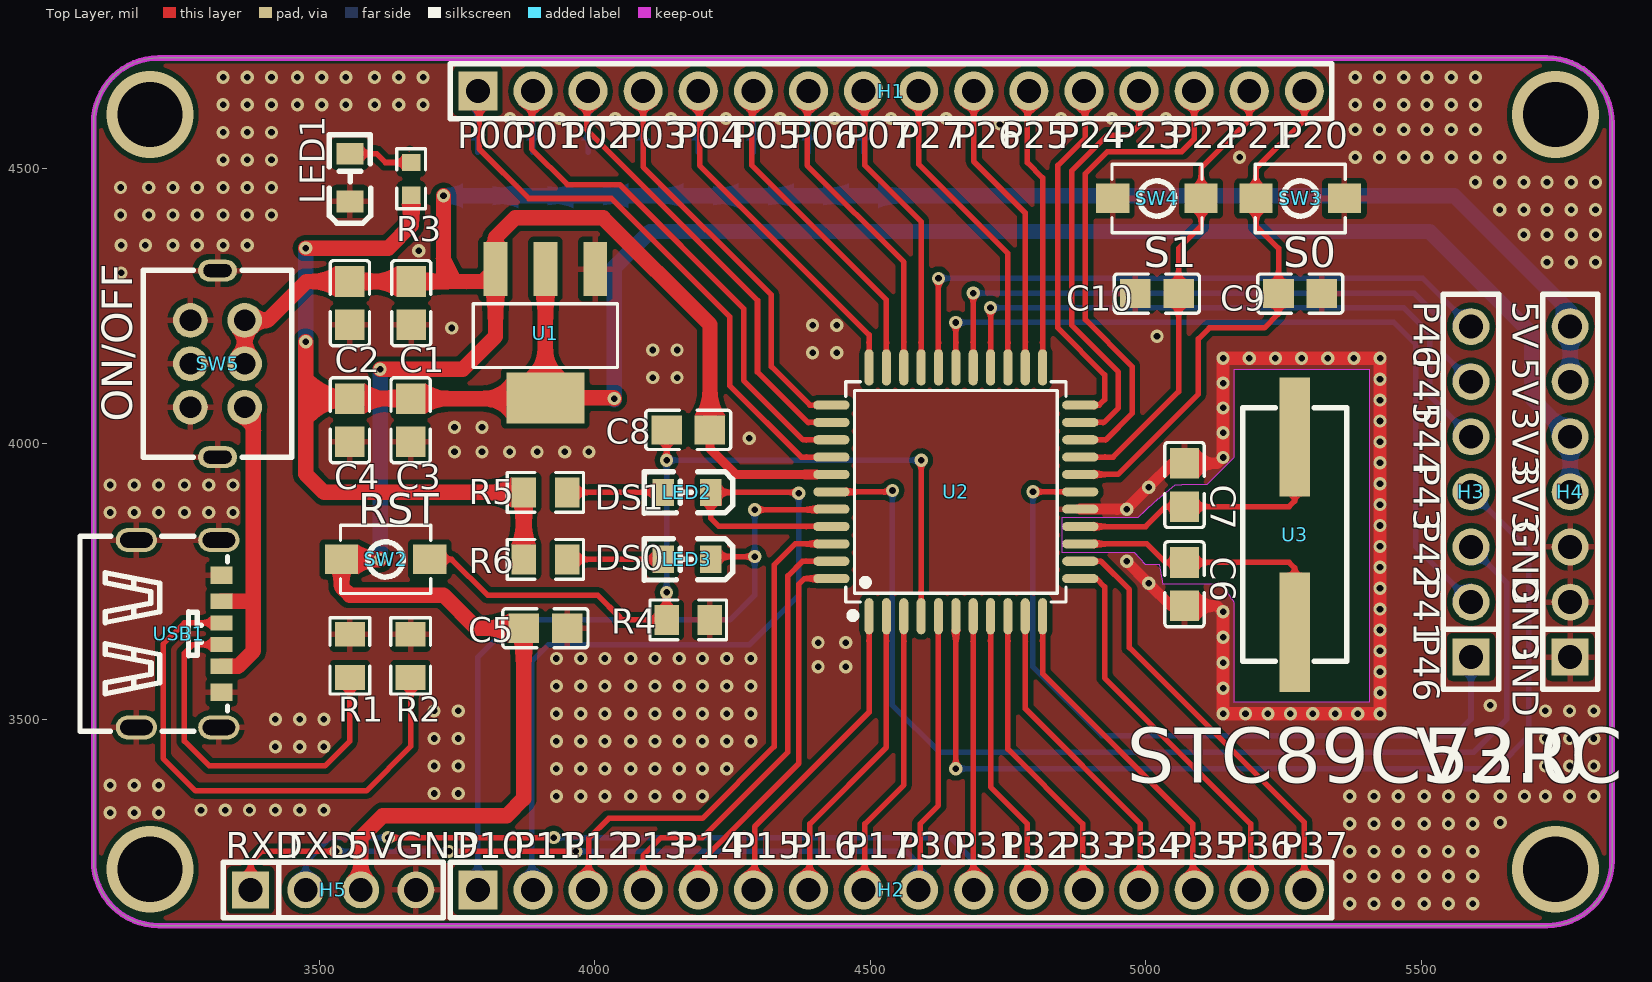
[diagram p0: Top Layer view]
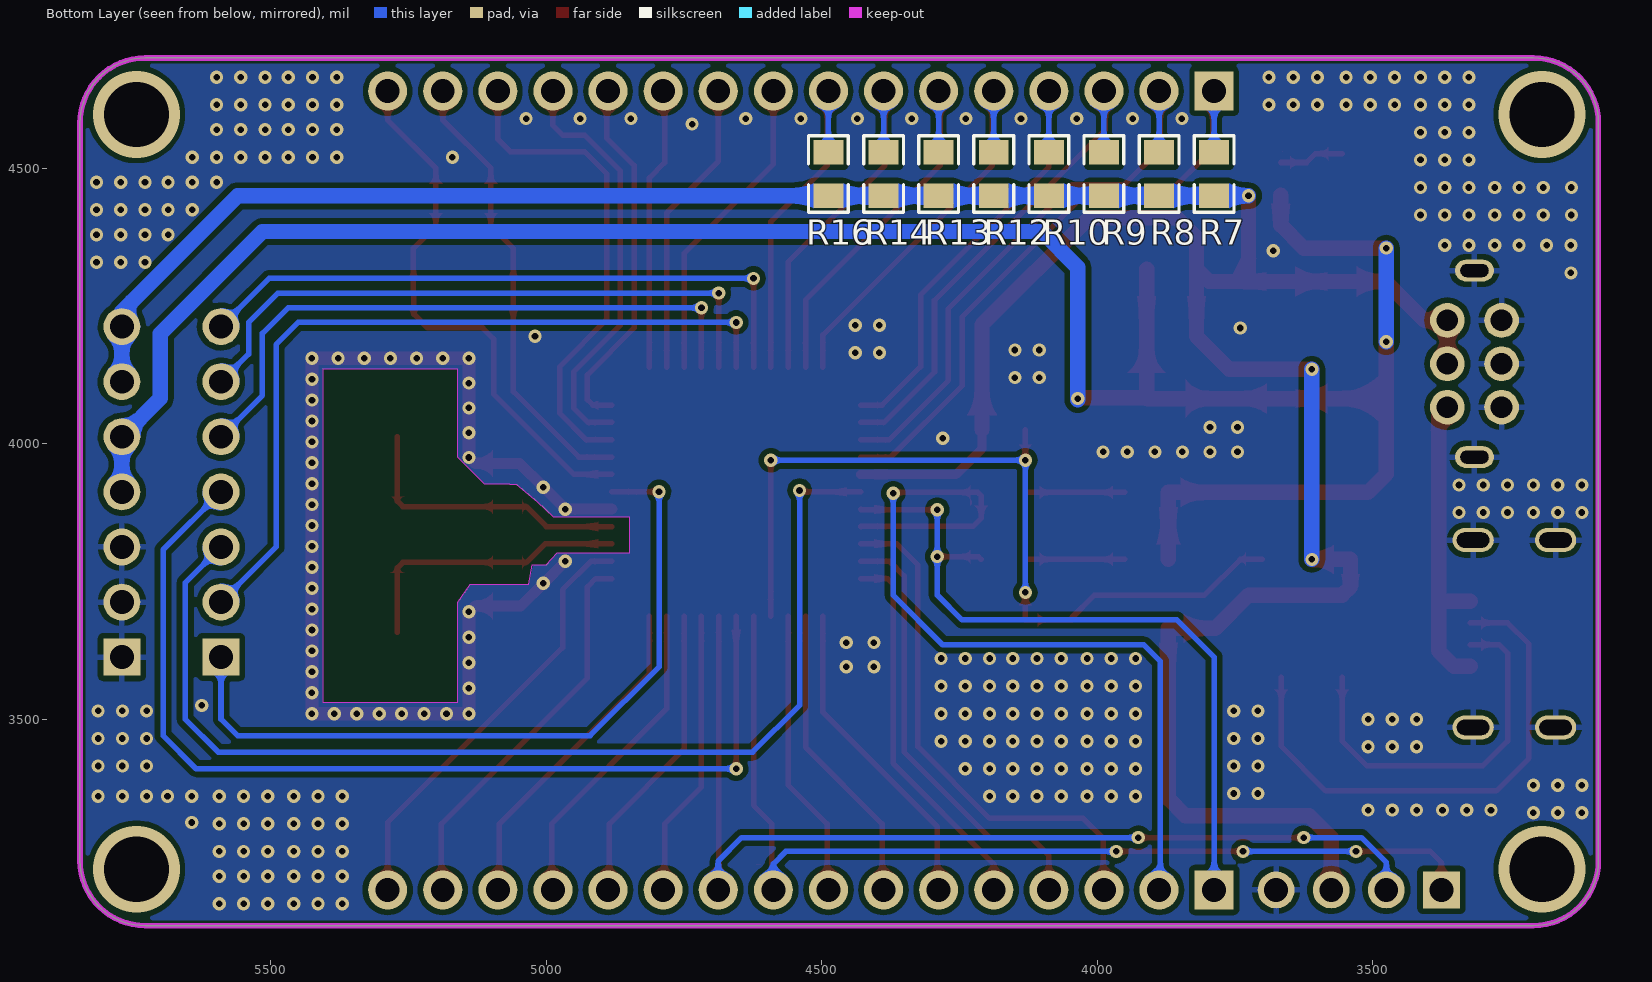
[diagram p1: Bottom Layer view, seen from below]
# Altium PCB MISC51716.pcbdoc
Units mil, origin at the board's own origin, x right, y up, seen from the top; angles counter-clockwise.
Board outline 2755.91 x 1574.8 mil, 2 copper layers (Top Layer, Bottom Layer), stack 62.206 mil thick; 40 components, 52 nets, 178 pads, 332 vias.

## Layer stack, top to bottom
Top Solder Mask Layer: solder mask 0.394, Dk 3.3
Top Layer: signal copper 1.379
Dielectric1: surface 59.449, FR4, Dk 4.5
Bottom Layer: signal copper 1.378
Bottom Solder Mask Layer: solder mask 0.394, Dk 3.3

## Board outline
3208.11,4700 ccw(c3208.11,4581.89) 3090,4581.89 3090,3243.31 ccw(c3208.11,3243.31) 3208.11,3125.2 5727.8,3125.2 ccw(c5727.8,3243.31) 5845.91,3243.31 5845.91,4581.89 ccw(c5727.8,4581.89) 5727.8,4700

## Design rules (kind name [scope] priority, off if disabled: settings)
BoardOutlineClearance copperThickness2oz_1 [All] p2 off: genericclearance=7.99 ignorepadtopadclearanceinfootprint=FALSE except(0: Arc-SplitContinuation Track-SplitContinuation SMDPad-SplitContinuation THPad-SplitContinuation Via-SplitContinuation Fill-SplitContinuation Region-SplitContinuation Poly-SplitContinuation Text-SplitContinuation Hole-SplitContinuation; 5.98: Arc-CutoutEdge SMDPad-CutoutEdge THPad-CutoutEdge Via-CutoutEdge Fill-CutoutEdge Region-CutoutEdge Text-CutoutEdge; 6.93: Hole-OutlineEdge Hole-CutoutEdge; 10: Poly-OutlineEdge Poly-CutoutEdge; 11.81: Arc-OutlineEdge Track-OutlineEdge SMDPad-OutlineEdge THPad-OutlineEdge Via-OutlineEdge Fill-OutlineEdge Region-OutlineEdge Text-OutlineEdge Track-CutoutEdge)
BoardOutlineClearance copperThickness1oz_1 [All] p4: genericclearance=4.02 ignorepadtopadclearanceinfootprint=FALSE except(0: Arc-SplitContinuation Track-SplitContinuation SMDPad-SplitContinuation THPad-SplitContinuation Via-SplitContinuation Fill-SplitContinuation Region-SplitContinuation Poly-SplitContinuation Text-SplitContinuation Hole-SplitContinuation; 6: SMDPad-CutoutEdge THPad-CutoutEdge Via-CutoutEdge Fill-CutoutEdge Region-CutoutEdge Text-CutoutEdge; 6.93: Hole-OutlineEdge Hole-CutoutEdge; 10: Poly-OutlineEdge Poly-CutoutEdge; 11.8: Arc-OutlineEdge Track-OutlineEdge SMDPad-OutlineEdge THPad-OutlineEdge Via-OutlineEdge Fill-OutlineEdge Region-OutlineEdge Text-OutlineEdge; 11.81: Arc-CutoutEdge Track-CutoutEdge)
Clearance copperThickness2oz [All] p1 off: gap=7.99 ignorepadtopadclearanceinfootprint=FALSE except(5.98: SMDPad-Track SMDPad-SMDPad THPad-Track SMDPad-THPad THPad-THPad Track-Via SMDPad-Via THPad-Via Via-Via Fill-Track Region-Track Fill-SMDPad Region-SMDPad Fill-THPad Region-THPad Fill-Via Region-Via Fill-Fill Fill-Region Region-Region Arc-Track Arc-SMDPad Arc-THPad Arc-Via Fill-Arc Region-Arc Arc-Arc Text-Track SMDPad-Text Text-THPad Text-Via Fill-Text Region-Text Arc-Text Text-Text; 6.93: Hole-Track Hole-SMDPad Hole-THPad Hole-Via Fill-Hole Region-Hole Hole-Arc Hole-Text; 10: Poly-Track Poly-SMDPad Poly-THPad Poly-Via Poly-Fill Poly-Region Poly-Poly Poly-Arc Poly-Text Poly-Hole)
Clearance copperThickness1oz [All] p3: gap=4.02 ignorepadtopadclearanceinfootprint=FALSE except(5.98: SMDPad-Track SMDPad-SMDPad THPad-Track SMDPad-THPad THPad-THPad Track-Via SMDPad-Via THPad-Via Via-Via Fill-Track Region-Track Fill-SMDPad Region-SMDPad Fill-THPad Region-THPad Fill-Via Region-Via Fill-Fill Fill-Region Region-Region; 6: Arc-Track Arc-SMDPad Arc-THPad Arc-Via Fill-Arc Region-Arc Arc-Arc Text-Track SMDPad-Text Text-THPad Text-Via Fill-Text Region-Text Arc-Text Text-Text; 6.93: Hole-Track Hole-SMDPad Hole-THPad Hole-Via Fill-Hole Region-Hole Hole-Arc Hole-Text; 10: Poly-Track Poly-SMDPad Poly-THPad Poly-Via Poly-Fill Poly-Region Poly-Poly Poly-Arc Poly-Text Poly-Hole)
Creepage creepage [All] p1: checkdistance=0 ignoreinternallayers=TRUE applytopolygonpour=TRUE
DiffPairsRouting differentialPair [All] p1: maxlimit=6 minlimit=6 mostfreqgap=6 toplayer_minwidth=5 toplayer_prefwidth=10 toplayer_maxwidth=100 toplayer_mingap=6 toplayer_prefgap=6 toplayer_maxgap=6 bottomlayer_minwidth=5 bottomlayer_prefwidth=10 bottomlayer_maxwidth=100 bottomlayer_mingap=6 bottomlayer_prefgap=6 bottomlayer_maxgap=6 maxuncoupledlength=10
HoleToHoleClearance otherClearance [All] p1: gap=11.81 allowstackedmicrovias=TRUE
Length netLength [All] p1: minlimit=0 maxlimit=0
MatchedLengths netLengthTolerance [All] p1: tolerance=1000
PasteMaskExpansion pasteMaskExpansion [All] p1: expansion=0
PlaneConnect innerPlane [All] p1: planeconnectstyle=Relief reliefexpansion=20 reliefentries=4 reliefconductorwidth=10 reliefairgap=10
PolygonConnect copperRegion [All] p1: connectstyle=Relief reliefconductorwidth=10 reliefentries=4 polygonreliefangle="90 Angle" airgapwidth=10 via.connectstyle=Relief via.reliefconductorwidth=10 via.reliefentries=4 via.polygonreliefangle="90 Angle" via.airgapwidth=10
RoutingVias viaSize [All] p1: holewidth=12.01 width=24.02 viastyle="Through Hole" minholewidth=11.81 minwidth=19.68 maxholewidth=248.03 maxwidth=393.7
SolderMaskExpansion solderMaskExpansion [IsVia] p1: expansion=-1000 istentingtop=TRUE
SolderMaskExpansion solderMaskExpansion [All] p2: expansion=2 istentingtop=FALSE
Width copperThickness2oz_2 [All] p1 off: maxlimit=100 minlimit=8 preferedwidth=10
Width copperThickness1oz_2 [All] p2: maxlimit=100 minlimit=5 preferedwidth=10

## Components (designator, comment, footprint, x,y, rotation, side; value= is the part's Value field where it differs from the comment)
C1 "100nF" C0805 3666.52,4255 r90 top
C2 "10UF" C0805 3555.15,4255 r90 top
C3 "100nF" C0805 3665.49,4042.5 r90 top
C4 "10UF" C0805 3555.15,4042.5 r90 top
C5 "100nF" C0805 3910,3665 r180 top
C6 "47PF" C0805 5070,3745 r270 top
C7 "47PF" C0805 5070,3925 r90 top
C8 "10UF" C0805 4169.33,4025 r180 top
C9 "10UF" C0805 5280,4272.5 r180 top
C10 "10UF" C0805 5020,4272.5 r0 top
H1 "" HDR-TH_16P-P2.54-V-M 4537.5,4640 r0 top
H2 "" HDR-TH_16P-P2.54-V-M 4537.5,3190 r0 top
H3 "" HDR-TH_7P-P2.54-V-M 5590,3912.5 r90 top
H4 "" HDR-TH_7P-P2.54-V-M 5770,3912.5 r90 top
H5 "" HDR-TH_4P-P2.54-V-M 3525,3190 r0 top
LED1 "" LED_0805 3555.55,4485 r90 top
LED2 "" LED_0805 4165,3911.91 r180 top
LED3 "" LED_0805 4165,3790.4 r180 top
R1 "5.1k" R0805 3555.15,3615 r90 top
R2 "5.1k" R0805 3665.49,3615 r90 top
R3 "1K" R0603 3666.52,4480.67 r90 top
R4 "10K" R0805 4169.33,3680 r180 top
R5 "1K" R0805 3910,3911.52 r180 top
R6 "1K" R0805 3910,3790 r180 top
R7 "10K" R0805 3787.5,4489.32 r90 bottom
R8 "10K" R0805 3887.5,4489.32 r90 bottom
R9 "10K" R0805 3987.5,4489.32 r90 bottom
R10 "10K" R0805 4087.5,4489.32 r90 bottom
R12 "10K" R0805 4187.5,4489.32 r90 bottom
R13 "10K" R0805 4287.5,4489.32 r90 bottom
R14 "10K" R0805 4387.5,4489.32 r90 bottom
R16 "10K" R0805 4487.5,4489.32 r90 bottom
SW2 "Tact switch 3*4*H" SW-SMD_L4.0-W2.9-LS5.0 3620,3790 r180 top
SW3 "Tact switch 3*4*H" SW-SMD_L4.0-W2.9-LS5.0 5280,4445 r0 top
SW4 "Tact switch 3*4*H" SW-SMD_L4.0-W2.9-LS5.0 5020,4445 r180 top
SW5 "SS22D03L6" SW-TH_SS-22D03-L4 3315,4145 r270 top
U1 "AMS1117-3.3" SOT-223-3_L6.5-W3.4-P2.30-LS7.0-BR 3910,4200 r90 top
U2 "STC89C52RC" LQFP-44_L10.0-W10.0-P0.80-LS12.0-BL 4655,3912.6 r0 top
U3 "12MHz" CRYSTAL-SMD_L11.4-W4.7-LS12.7 5270,3835 r270 top
USB1 "TYPE_C_SMD_6P" TYPE-C-SMD_TYPE-C-6P 3245,3655 r270 top

## Footprints (in the part's own frame and the unit in brackets; to place one, negate y for a bottom-side part, rotate by r counter-clockwise, add the part's x,y. Pads: shape width x height; smd on the part's side, far side on the other; paste and mask are expansions set on the pad)
C0805 [mm]
  rect 1.41x1.35 smd paste-100 mask+0.051: 1(-1,0) 2(1,0)
  silkscreen extent -1.96,-0.9 1.96,0.9
CRYSTAL-SMD_L11.4-W4.7-LS12.7 [mm]
  rect 5.5x1.4 smd: 1(-4.5,0) 2(4.5,0)
  silkscreen extent -5.85,-2.4 5.85,2.4
HDR-TH_4P-P2.54-V-M [mm]
  rect 1.7x1.7 hole 1.1: 1(-3.81,0)
  round 1.7 hole 1.1: 2(-1.27,0) 3(1.27,0) 4(3.81,0)
  silkscreen extent -5.08,-1.27 5.08,1.27
HDR-TH_7P-P2.54-V-M [mm]
  rect 1.7x1.7 hole 1.1: 1(-7.62,0)
  round 1.7 hole 1.1: 2(-5.08,0) 3(-2.54,0) 4(0,0) 5(2.54,0) 6(5.08,0) 7(7.62,0)
  silkscreen extent -9.1,-1.27 9.1,1.27
HDR-TH_16P-P2.54-V-M [mm]
  rect 1.8x1.8 hole 1.1: 1(-19.05,0)
  round 1.8 hole 1.1: 2(-16.51,0) 3(-13.97,0) 4(-11.43,0) 5(-8.89,0) 6(-6.35,0) 7(-3.81,0) 8(-1.27,0) 9(1.27,0) 10(3.81,0) 11(6.35,0) 12(8.89,0) 13(11.43,0) 14(13.97,0) 15(16.51,0) 16(19.05,0)
  silkscreen extent -20.32,-1.27 20.32,1.27
LED_0805 [mm]
  rect 1x1.25 smd paste+0 mask+0.051: 1(-1.15,0.005) 2(1.05,0.005)
  silkscreen extent -2.15,-0.94 1.93,0.97
LQFP-44_L10.0-W10.0-P0.80-LS12.0-BL [mm]
  oval 0.42x1.67 smd: 1(-4,-5.735) 2(-3.2,-5.735) 3(-2.4,-5.735) 4(-1.6,-5.735) 5(-0.8,-5.735) 6(0,-5.735) 7(0.8,-5.735) 8(1.6,-5.735) 9(2.4,-5.735) 10(3.2,-5.735) 11(4,-5.735) 23(4,5.735) 24(3.2,5.735) 25(2.4,5.735) 26(1.6,5.735) 27(0.8,5.735) 28(0,5.735) 29(-0.8,5.735) 30(-1.6,5.735) 31(-2.4,5.735) 32(-3.2,5.735) 33(-4,5.735)
  oval 1.67x0.42 smd: 12(5.735,-4) 13(5.735,-3.2) 14(5.735,-2.4) 15(5.735,-1.6) 16(5.735,-0.8) 17(5.735,0) 18(5.735,0.8) 19(5.735,1.6) 20(5.735,2.4) 21(5.735,3.2) 22(5.735,4) 34(-5.735,4) 35(-5.735,3.2) 36(-5.735,2.4) 37(-5.735,1.6) 38(-5.735,0.8) 39(-5.735,0) 40(-5.735,-0.8) 41(-5.735,-1.6) 42(-5.735,-2.4) 43(-5.735,-3.2) 44(-5.735,-4)
  silkscreen extent -5.08,-5.85 5.08,5.08
R0603 [mil]
  rect 31.75x34.02 smd paste-3937.01 mask+2: 1(-29.66,0) 2(29.66,0)
  silkscreen extent -55,-26 55,26
R0805 [mm]
  rect 1.133x1.377 smd paste-100 mask+0.051: 1(-1,0) 2(1,0)
  silkscreen extent -1.76,-0.92 1.76,0.92
SOT-223-3_L6.5-W3.4-P2.30-LS7.0-BR [mm]
  rect 2.5x1.1 smd: 1(2.97,-2.3) 2(2.97,0) 3(2.97,2.3)
  rect 2.34x3.6 smd: 4(-2.97,0)
  silkscreen extent -1.57,-3.33 1.37,3.33
SW-SMD_L4.0-W2.9-LS5.0 [mm]
  rect 1.53x1.36 smd: 1(-2.035,0) 2(2.035,0)
  silkscreen extent -2.08,-1.58 2.08,1.58
SW-TH_SS-22D03-L4 [mm]
  round 1.6 hole 1: 1(-2,-1.25) 2(0,-1.25) 3(2,-1.25) 4(-2,1.25) 5(0,1.25) 6(2,1.25)
  oval 1x1.8 hole 0.6 slot 1.3 at 90 deg: 7(-4.3,0) 8(4.3,0)
  silkscreen extent -4.32,-3.43 4.32,3.43
TYPE-C-SMD_TYPE-C-6P [mm]
  oval 1.1x1.9 hole 0.7 slot 1.5 at 90 deg: 7(-4.32,-1.963) 7(-4.32,1.838) 7(4.32,-1.963) 7(4.32,1.838)
  rect 0.7x1 smd paste-100 mask+0.051: A5(-0.5,1.963) A9(1.5,1.963) B5(0.5,1.963) B9(-1.5,1.963)
  rect 0.8x1 smd paste-100 mask+0.051: A12(2.7,1.963) B12(-2.7,1.963)
  silkscreen extent -4.5,-4.56 4.5,2.24

## Via types
v1: diameter 24, hole 12, Top Layer to Bottom Layer, 328 vias
v2: diameter 157.48, hole 118.1, Top Layer to Bottom Layer, 4 vias

## Nets (pads, with @x,y where several pads share a name; then routed paths per layer and width w, separated by ;. In a path a pad name is that pad's centre, name@x,y a point inside that pad or via, vN(x,y) a via of type N, cw(c..) or ccw(c..) an arc to the next point about the centre after c; other vN are vias at no path point)
3.3V: C3.2 C4.2 H4.4 H4.5 R3.1 R5.2 R6.2 U1.2 U1.4 | length 4326.1
  Top Layer w27.9: v1(3475,4185) 3475,4077.05 ; v1(3475,4355) 3625,4355 3666.52,4396.52 R3.1 ; R6.2 R5.2 3508.48,3911.52 3475,3945 3475,4077.05 ; U1.2 U1.4 ; v1(4035,4081.87) 4033.8,4083.07 U1.4 ; 3475,4077.05 3479.82,4081.87 C4.2 C3.2 3908.8,4081.87 U1.4
  Bottom Layer w27.9: v1(3475,4185) v1(3475,4355) ; v1@4035,4080 4035,4320 4100,4385 5515,4385 5700,4200 5700,4082.5 H4.5 H4.4
$1N13: LED1.2 R3.2 | length 117.8
  Top Layer w10: LED1.2 3603.66,4526.34 3619.67,4510.33 R3.2
$1N16: LED3.2 R6.1 | length 174.4
  Top Layer w10: R6.1 4123.47,3790 LED3.2
$1N17: LED2.2 R5.1 | length 174.4
  Top Layer w10: R5.1 4123.47,3911.52 LED2.2
$1N128: R2.1 USB1.A5 | length 961.6
  Top Layer w10: USB1.A5 3254.68,3674.68 3216.14,3636.14 3216.14,3428.86 3275,3370 3585,3370 3665.49,3450.49 R2.1
$1N129: R1.1 USB1.B5 | length 686.6
  Top Layer w10: USB1.B5 3270.32,3635.32 3255,3620 3255,3460 3300,3415 3510,3415 3555,3460 3555,3575.48 R1.1
$1N7753: 
+5V: C1.2 C2.2 C5.2 C8.1 H4.6 H4.7 H5.3 R7.1 R8.1 R9.1 R10.1 R12.1 R13.1 R14.1 R16.1 SW2.2 SW5.4 SW5.5 U1.3 U2.38 | length 5907.1
  Top Layer w16.5: C8.1 4208.7,3991.3 4255.9,3944.1 U2.38
  Top Layer w27.9: SW5.5 SW5.4 3405.39,4223.73 3476.03,4294.37 C2.2 C1.2 3725,4294.37 ; H5.3 3575,3285 3615,3325 3840,3325 3870.63,3355.63 C5.2 3785,3665 3725,3725 3555,3725 3539.88,3740.12 SW2.2 v1(3610,3790) ; v1(3610,4135) 3760,4135 3819.45,4194.45 U1.3 ; v1(3725,4450) 3725,4294.37 ; C8.1 4208.7,4216.3 4015,4410 3855,4410 3819.45,4374.45 U1.3 ; 3725,4294.37 3796.89,4294.37 U1.3
  Bottom Layer w27.9: v1(3610,3790) v1(3610,4135) ; v1(3725,4450) R7.1 R8.1 R9.1 R10.1 R12.1 R13.1 R14.1 R16.1 ; R16.1 5560.05,4449.95 5770,4240 H4.7 H4.6
GND: C1.1 C2.1 C3.1 C4.1 C5.1 C6.2 C7.2 C9.1 C10.1 H4.1 H4.2 H4.3 H5.4 LED1.1 R1.2 R2.2 R4.1 SW3.2 SW4.2 SW5.1 SW5.2 SW5.3 SW5.7 SW5.8 U1.1 U2.16 USB1.7 USB1.A12 USB1.B12 | length 2091
  Top Layer w20: U2.16 v1(4965,3881.1) v1(5005,3921.1) 5048.27,3964.37 C7.2 5129.37,3964.37 v1(5140,3975) ; v1(4965,3786.6) v1(5005,3746.6) 5045.97,3705.63 C6.2 5129.37,3705.63 v1(5140,3695)
  Top Layer w24: v1(5140,3695) v1(5140,3648.75) v1(5140,3602.5) v1(5140,3556.25) v1(5140,3510) v1(5180.71,3510) v1(5221.43,3510) v1(5262.14,3510) v1(5302.86,3510) v1(5343.57,3510) v1(5384.29,3510) v1(5425,3510) v1(5425,3547.94) v1(5425,4155) v1(5377.5,4155) v1(5330,4155) v1(5282.5,4155) v1(5235,4155) v1(5187.5,4155) v1(5140,4155) v1(5140,4110) v1(5140,4065) v1(5140,4020) v1(5140,3975)
  other v1: 5370,3165 5414,3165 5458,3165 5505,3165 5549,3165 5593,3165 5370,3215 5414,3215 5458,3215 5505,3215 5549,3215 5593,3215 5370,3260 5414,3260 5458,3260 5505,3260 5549,3260 5593,3260 5370,3310 5414,3310 5458,3310 5505,3310 5549,3310 5593,3310 5643,3312.5 3120,3330 3164,3330 3208,3330 3285,3335 3329,3335 3373,3335 3420,3335 3464,3335 3508,3335 3930,3360 3974,3360 4018,3360 4065,3360 4109,3360 4153,3360 4195,3360 5370,3360 5414,3360 5458,3360 5505,3360 5549,3360 5593,3360 5643,3360 5687,3360 5725,3360 5769,3360 5813,3360 3708,3365 3752,3365 3120,3380 3164,3380 3208,3380 3930,3410 3974,3410 4018,3410 4065,3410 4109,3410 4153,3410 4195,3410 4239,3410 3708,3415 3752,3415 5725,3415 5769,3415 5813,3415 3420,3450 3464,3450 3508,3450 3930,3460 3974,3460 4018,3460 4065,3460 4109,3460 4153,3460 4195,3460 4239,3460 4283,3460 3708,3465 3752,3465 5725,3465 5769,3465 5813,3465 3420,3500 3464,3500 3508,3500 3930,3510 3974,3510 4018,3510 4065,3510 4109,3510 4153,3510 4195,3510 4239,3510 4283,3510 3708,3515 3752,3515 5725,3515 5769,3515 5813,3515 5625,3525 3930,3560 3974,3560 4018,3560 4065,3560 4109,3560 4153,3560 4195,3560 4239,3560 4283,3560 5424.88,3585.88 4405,3595 4455,3595 3930,3610 3974,3610 4018,3610 4065,3610 4109,3610 4153,3610 4195,3610 4239,3610 4283,3610 5424.88,3623.82 4405,3639 4455,3639 5424.88,3661.76 5424.88,3699.71 5424.88,3737.65 5424.88,3775.59 5424.88,3813.53 5424.88,3851.47 3120,3875 3164,3875 3208,3875 3255,3875 3299,3875 3343,3875 5424.88,3889.41 3120,3925 3164,3925 3208,3925 3255,3925 3299,3925 3343,3925 5424.88,3927.35 5424.88,3965.29 3745,3985 3795,3985 3845,3985 3895,3985 3945,3985 3989,3985 5424.88,4003.24 4280,4010 3745,4030 3795,4030 5424.88,4041.18 5424.88,4079.12 5424.88,4117.06 4105,4120 4149,4120 4395,4165 4439,4165 4105,4170 4149,4170 5020,4195 3740,4210 4395,4215 4439,4215 3140,4310 5728,4329.4 5772,4329.4 5816,4329.4 3680,4350 3140,4360 3184,4360 3234,4360 3278,4360 3325,4360 3369,4360 5686,4379.4 5728,4379.4 5772,4379.4 5816,4379.4 3139,4415 3190,4415 3234,4415 3278,4415 3325,4415 3369,4415 3413,4415 5642,4424.4 5686,4424.4 5728,4424.4 5772,4424.4 5816,4424.4 3139,4465 3190,4465 3234,4465 3278,4465 3325,4465 3369,4465 3413,4465 5598,4474.4 5642,4474.4 5686,4474.4 5728,4474.4 5772,4474.4 5816,4474.4 3325,4515 3369,4515 3413,4515 5170,4520 5380,4520 5424,4520 5468,4520 5510,4520 5554,4520 5598,4520 5642,4520 3325,4565 3369,4565 3413,4565 5380,4570 5424,4570 5468,4570 5510,4570 5554,4570 5598,4570 4735,4580 3846.02,4590 3935.49,4590 4036.73,4590 4137.97,4590 4238.03,4590 4336.33,4590 4435,4590 4537.5,4590 4637.4,4590 4845.96,4590 4938.18,4590 5036.28,4590 3325,4615 3369,4615 3413,4615 3460,4615 3504,4615 3548,4615 3600,4615 3644,4615 3688,4615 5380,4615 5424,4615 5468,4615 5510,4615 5554,4615 5598,4615 3325,4665 3369,4665 3413,4665 3460,4665 3504,4665 3548,4665 3600,4665 3644,4665 3688,4665 5380,4665 5424,4665 5468,4665 5510,4665 5554,4665 5598,4665
P0.0: H1.1 R7.2 U2.37 | length 1161.5
  Top Layer w10: H1.1 3790,4637.5 3790,4535 3880,4445 4030,4445 4245,4230 4245,4105 4374.41,3975.59 U2.37
  Bottom Layer w10: R7.2 H1.1
P0.1: H1.2 R8.2 U2.36 | length 1056.4
  Top Layer w10: H1.2 3885,4637.5 3885,4535 3950,4470 4045,4470 4270,4245 4270,4115 4377.91,4007.09 U2.36
  Bottom Layer w10: R8.2 H1.2
P0.2: H1.3 R9.2 U2.35 | length 922.8
  Top Layer w10: H1.3 3985,4637.5 3985,4570 4295,4260 4295,4130 4386.42,4038.58 U2.35
  Bottom Layer w10: R9.2 H1.3
P0.3: H1.4 R10.2 U2.34 | length 845.8
  Top Layer w10: H1.4 4087.5,4502.5 4320,4270 4320,4140 4389.92,4070.08 U2.34
  Bottom Layer w10: R10.2 H1.4
P0.4: H1.5 R12.2 U2.33 | length 741.3
  Top Layer w10: H1.5 4190,4637.5 4190,4505 4497.52,4197.48 U2.33
  Bottom Layer w10: R12.2 H1.5
P0.5: H1.6 R13.2 U2.32 | length 715
  Top Layer w10: H1.6 4285,4637.5 4285,4505 4529.02,4260.98 U2.32
  Bottom Layer w10: R13.2 H1.6
P0.6: H1.7 R14.2 U2.31 | length 686.7
  Top Layer w10: H1.7 4385,4637.5 4385,4505 4560.51,4329.49 U2.31
  Bottom Layer w10: R14.2 H1.7
P0.7: H1.8 R16.2 U2.30 | length 656.2
  Top Layer w10: H1.8 4490,4637.5 4490,4505 4592.01,4402.99 U2.30
  Bottom Layer w10: R16.2 H1.8
P1.0: H2.1 LED3.1 U2.40 | length 1348
  Top Layer w10: LED3.1 4215.09,3795 v1(4290,3795) ; v1(4290,3880) 4428.11,3880 U2.40
  Bottom Layer w10: H2.1 3787.5,3612.5 3855,3680 4245,3680 4290,3725 v1(4290,3795) v1(4290,3880)
P1.1: H2.2 LED2.1 U2.41 | length 1564.8
  Top Layer w10: v1(4370,3910) 4368.29,3911.71 4216.71,3911.71 4210,3905 4210,3865 4225,3850 4428.82,3850 U2.41
  Bottom Layer w10: H2.2 3885,3192.5 3885,3605 3915,3635 4280,3635 4370,3725 v1(4370,3910)
P1.2: H2.3 U2.42 | length 951.4
  Top Layer w10: H2.3@3982.5,3190 3988.97,3196.47 3988.97,3283.97 4025,3320 4195,3320 4325,3450 4325,3780 4363.11,3818.11 U2.42
P1.3: H2.4 U2.43 | length 812.9
  Top Layer w10: H2.4 4087.5,3252.5 4120,3285 4195,3285 4350,3440 4350,3760 4376.62,3786.62 U2.43
P1.4: H2.5 U2.44 | length 694.1
  Top Layer w10: H2.5 4187.5,3237.5 4370,3420 4370,3745.12 4380,3755.12 U2.44
P1.5: H2.6 U2.1 | length 583.8
  Top Layer w10: H2.6 4290,3192.5 4290,3305 4497.52,3512.52 U2.1
P1.6: H2.7 U2.2 | length 555.4
  Top Layer w10: H2.7 4390,3192.5 4390,3310 4529.02,3449.02 U2.2
P1.7: H2.8 U2.3 | length 527.1
  Top Layer w10: H2.8 4490,3192.5 4490,3310 4560.51,3380.51 U2.3
P2.0: C9.2 H1.16 SW3.1 U2.18 | length 996.7
  Top Layer w10: U2.18 4949.1,3944.1 5095,4090 5095,4190 5115,4210 5215,4210 5240,4235 5240,4271.87 C9.2 5240.63,4354.37 5200,4395 5200,4444.88 SW3.1 5199.88,4499.88 5287.5,4587.5 H1.16
P2.1: C10.2 H1.15 SW4.1 U2.19 | length 826.5
  Top Layer w10: U2.19 4940.59,3975.59 5059.37,4094.37 C10.2 5059.37,4354.37 5100.12,4395.12 SW4.1 5100.12,4500.12 5187.5,4587.5 H1.15
P2.2: H1.14 U2.20 | length 895.2
  Top Layer w10: U2.20 4927.09,4007.09 4975,4055 4975,4140 4890,4225 4890,4490 4930,4530 5065,4530 5087.5,4552.5 H1.14
P2.3: H1.13 U2.21 | length 764.5
  Top Layer w10: U2.21 4923.58,4038.58 4950,4065 4950,4130 4865,4215 4865,4495 4930,4560 4970,4560 4987.5,4577.5 H1.13
P2.4: H1.12 U2.22 | length 665.2
  Top Layer w10: U2.22 4915,4070.08 4925,4080.08 4925,4125 4840,4210 4840,4505 4890,4555 4890,4637.5 H1.12
P2.5: H1.11 U2.23 | length 514
  Top Layer w10: H1.11 4785,4637.5 4785,4510 4812.48,4482.52 U2.23
P2.6: H1.10 U2.24 | length 540.3
  Top Layer w10: H1.10 4687.5,4512.5 4780.98,4419.02 U2.24
P2.7: H1.9 U2.25 | length 568.7
  Top Layer w10: H1.9 4587.5,4507.5 4749.49,4345.51 U2.25
P3.0: H2.9 H5.1 U2.5 | length 1839.3
  Top Layer w10: H5.1 3375,3240 3395,3260 v1(3530,3260) ; v1(3735,3260) v1(3965,3260) ; H2.9 4590,3192.5 4590,3310 4623.5,3343.5 U2.5
  Bottom Layer w10: v1(3530,3260) v1(3735,3260) ; v1(3965,3260) 4565,3260 4587.5,3237.5 H2.9
P3.1: H2.10 H5.2 U2.7 | length 1848.5
  Top Layer w10: v1(3625,3285) v1(3925,3285) ; U2.7 4686.5,3191 H2.10
  Bottom Layer w10: H5.2 3475,3240 3520,3285 v1(3625,3285) ; v1(3925,3285) 4645,3285 4687.5,3242.5 H2.10
P3.2: H2.11 U2.8 | length 525.6
  Top Layer w10: U2.8 4717.99,3377.01 4785,3310 4785,3192.5 H2.11
P3.3: H2.12 U2.9 | length 554
  Top Layer w10: U2.9 4749.49,3445.51 4885,3310 4885,3192.5 H2.12
P3.4: H2.13 U2.10 | length 584.4
  Top Layer w10: U2.10 4780.98,3519.02 4990,3310 4990,3192.5 H2.13
P3.5: H2.14 U2.11 | length 610.7
  Top Layer w10: U2.11 4812.48,3582.52 5085,3310 5085,3192.5 H2.14
P3.6: H2.15 U2.12 | length 711.3
  Top Layer w10: U2.12 4909.88,3755.12 4925,3740 4925,3575 5190,3310 5190,3192.5 H2.15
P3.7: H2.16 U2.13 | length 787.1
  Top Layer w10: U2.13 4918.38,3786.62 4970,3735 4970,3630 5287.5,3312.5 H2.16
P4.0: H3.1 U2.17 | length 1375.1
  Top Layer w10: v1(4795,3912.6) U2.17
  Bottom Layer w10: v1(4795,3912.6) 4795,3595 4920,3470 5560,3470 5590,3500 H3.1
P4.1: H3.2 U2.28 | length 1442.1
  Top Layer w10: U2.28 v1(4655,4220)
  Bottom Layer w10: v1(4655,4220) 5450,4220 5490,4180 5490,3812.5 H3.2
P4.2: H3.3 U2.39 | length 2016.3
  Top Layer w10: U2.39 4537.6,3912.6 v1(4540,3915)
  Bottom Layer w10: v1(4540,3915) 4540,3525 4625,3440 5595,3440 5655,3500 5655,3747.5 H3.3
P4.3: H3.4 U2.6 | length 1827.7
  Top Layer w10: v1(4655,3410) U2.6
  Bottom Layer w10: v1(4655,3410) 5635,3410 5695,3470 5695,3807.5 H3.4
P4.4: H3.5 U2.26 | length 1141.5
  Top Layer w10: U2.26 v1@4717.99,4245
  Bottom Layer w10: v1(4717.99,4246.67) 5468.33,4246.67 5515,4200 5515,4087.5 H3.5
P4.5: H3.6 U2.27 | length 1140.4
  Top Layer w10: U2.27 v1@4686.5,4275
  Bottom Layer w10: v1(4686.5,4273.33) 5486.67,4273.33 5540,4220 5540,4162.5 H3.6
P4.6: H3.7 U2.29 | length 1164.4
  Top Layer w10: U2.29 v1(4623.5,4300)
  Bottom Layer w10: v1(4623.5,4300) 5502.5,4300 H3.7
RST: C8.2 R4.2 SW2.1 U2.4 | length 1568.5
  Top Layer w10: SW2.1 3740,3790 3805,3725 4005,3725 4045,3685 4045,3680 R4.2 ; v1(4130,3970) C8.2 ; R4.2 v1(4130,3730) ; U2.4 v1(4592.01,3970)
  Bottom Layer w10: v1(4130,3730) v1(4130,3970) v1(4592.01,3970)
VCC+5V: SW5.6 USB1.A9 USB1.B9 | length 576
  Top Layer w27.9: USB1.A9 3352.1,3595.95 3380,3623.84 3380,3714.05 ; USB1.B9 3380,3714.05 ; SW5.6 3380,4050.46 3380,3714.05
XTAL1: C7.1 U2.15 U3.1 | length 524.8
  Top Layer w10: U2.15 4999.61,3849.61 5035.63,3885.63 C7.1 5260,3885.63 5270,3895.63 U3.1
XTAL2: C6.1 U2.14 U3.2 | length 523.9
  Top Layer w10: U2.14 5001.89,3818.11 5035.63,3784.37 C6.1 5260,3784.37 5270,3774.37 U3.2
copper on no net:
  other v2: 3192.36,3227.56 5743.54,3227.56 3192.36,4597.64 5743.54,4597.64

## Polygon pours and split planes (outlines as drawn)
GND on Top Layer (solid, remove dead copper, pour order 0): 3045,4800 3045,3085 5930,3085 5930,4800
GND on Bottom Layer (solid, remove dead copper, pour order 4): 3000,4850 3000,3000 5990,3000 5990,4850

## Keep-outs
Board Outline Layer:
  region: 5405,3530.64 5160,3530.64 5160,3711.85 5137.49,3745 5031.8,3745 5024.76,3780 5000,3780 4979.82,3801.93 4848.03,3801.93 4848.03,3866.12 4986.24,3866.12 5015.25,3893.28 5053.44,3925 5065,3925 5066.28,3926.28 5111.28,3926.28 5160,3975 5160,4135.31 5405,4135.31
  lines w10: 3090,3243.31 3090,4581.89 cw(c3208.11,4581.89) 3208.11,4700 5727.8,4700 cw(c5727.8,4581.89) 5845.91,4581.89 5845.91,3243.31 cw(c5727.8,3243.31) 5727.8,3125.2 3208.11,3125.2 cw(c3208.11,3243.31) 3090,3243.31

## Other copper
Top Layer:
  drawing of 181 lines, arcs and shapes, not listed
Bottom Layer:
  drawing of 75 lines, arcs and shapes, not listed

## Silkscreen, mask and mechanical layers (free items; w line width, h text height)
Top Silkscreen Layer:
  text "P00" at 3750,4536.19 h48
  text "P01" at 3852.46,4536.19 h48
  text "P02" at 3942.81,4536.19 h48
  text "P03" at 4045.27,4536.19 h48
  text "P04" at 4147.73,4536.19 h48
  text "P05" at 4251.49,4536.19 h48
  text "P06" at 4353.94,4536.19 h48
  text "P07" at 4455,4536.19 h48
  text "P27" at 4550,4536.19 h48
  text "P26" at 4651.26,4536.19 h48
  text "P25" at 4738.71,4536.19 h48
  text "P24" at 4839.97,4536.19 h48
  text "P23" at 4941.23,4536.19 h48
  text "P22" at 5043.99,4536.19 h48
  text "P21" at 5145.24,4536.19 h48
  text "P20" at 5245,4536.19 h48
  text "S1" at 4995.8,4320 h55
  text "S0" at 5248.9,4320 h55
  text "P46" at 5486.19,4258.27 h48 r270
  text "5V" at 5666.19,4258.27 h48 r270
  text "P45" at 5486.19,4155.81 h48 r270
  text "5V" at 5666.19,4155.81 h48 r270
  text "P44" at 5486.19,4065.45 h48 r270
  text "3V3" at 5666.19,4065.45 h48 r270
  text "ON/OFF" at 3160,4040 h55 r90
  text "P43" at 5486.19,3963 h48 r270
  text "3V3" at 5666.19,3963 h48 r270
  text "DS1" at 4000,3880 h45
  text "P42" at 5486.19,3860.54 h48 r270
  text "GND" at 5666.19,3860.54 h48 r270
  text "RST" at 3570,3855 h55
  text "DS0" at 4000,3770 h45
  text "P41" at 5486.19,3756.78 h48 r270
  text "GND" at 5666.19,3756.78 h48 r270
  text "P46" at 5486.19,3654.33 h48 r270
  text "GND" at 5666.19,3654.33 h48 r270
  text "STC89C52RC" at 4965,3385 h100
  text "V3.0" at 5490,3385 h100
  text "RXD" at 3330,3247.5 h48
  text "TXD" at 3433,3247.5 h48
  text "5V" at 3550,3247.5 h48
  text "GND" at 3638,3247.5 h48
  text "P10" at 3750,3247.5 h48
  text "P11" at 3852.46,3247.5 h48
  text "P12" at 3942.8,3247.5 h48
  text "P13" at 4045.27,3247.5 h48
  text "P14" at 4147.73,3247.5 h48
  text "P15" at 4251.49,3247.5 h48
  text "P16" at 4353.94,3247.5 h48
  text "P17" at 4455,3247.5 h48
  text "P30" at 4550,3247.5 h48
  text "P31" at 4651.26,3247.5 h48
  text "P32" at 4738.71,3247.5 h48
  text "P33" at 4839.97,3247.5 h48
  text "P34" at 4941.23,3247.5 h48
  text "P35" at 5043.99,3247.5 h48
  text "P36" at 5145.24,3247.5 h48
  text "P37" at 5245,3247.5 h48